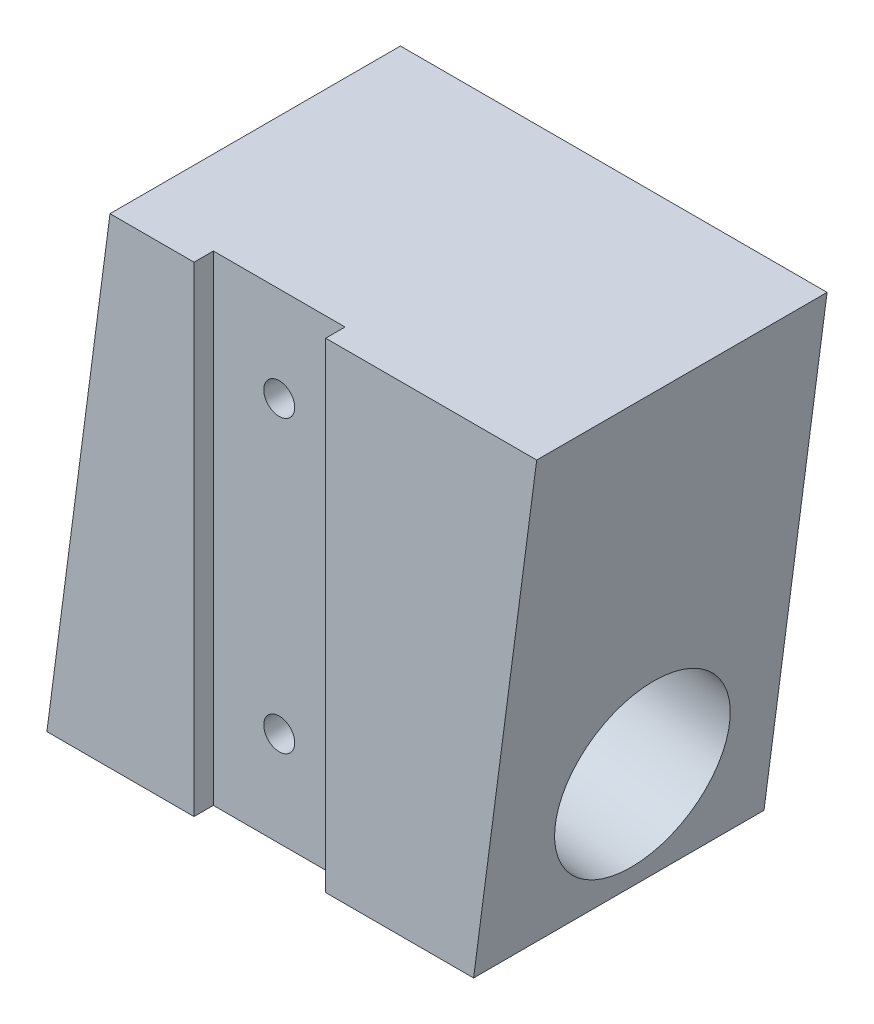
SolidWorks part; units mm, degrees
material "6061 合金"
ref_plane "前视基准面" through (0, 0, 0) normal (0, 0, 1) x (1, 0, 0)
ref_plane "上视基准面" through (0, 0, 0) normal (0, 1, 0) x (1, 0, 0)
ref_plane "右视基准面" through (0, 0, 0) normal (1, 0, 0) x (0, 0, -1)
sketch "草图1" plane through (0, 0, 0) normal (0, 0, 1) x (1, 0, 0)
  line L1 (-19.6362, 9.8181) -> (5.6638, 9.8181)
  line L2 (-19.6362, 9.8181) -> (-19.6362, -14.9819)
  line L3 (-19.6362, -14.9819) -> (5.6638, -14.9819)
  line L4 (5.6638, 9.8181) -> (5.6638, -14.9819)
  dimension "D1" = 24.8
  dimension "D2" = 25.3
extrude "凸台-拉伸1" add sketch "草图1" along normal blind 15
sketch "草图2" plane through (0, 0, 0) normal (0, 0, -1) x (-1, 0, 0)
  line L0 (-5.6638, 9.8181) -> (-2.4038, -14.9819)
  line L1 (19.6362, -14.9819) -> (-5.6638, -14.9819) construction
  line L2 (-2.4038, -14.9819) -> (-5.6638, -14.9819)
  line L3 (-5.6638, -14.9819) -> (-5.6638, 9.8181)
  line L4 (16.3762, 9.8181) -> (19.6362, 9.8181)
  line L5 (-5.6638, 9.8181) -> (19.6362, 9.8181) construction
  line L6 (19.6362, 9.8181) -> (19.6362, -14.9819)
  line L7 (19.6362, -14.9819) -> (16.3762, 9.8181)
  dimension "D1" = 3.26
  dimension "D2" = 3.26
extrude "切除-拉伸1" cut sketch "草图2" against normal up to next
sketch "草图3" plane through (0, -14.9819, 0) normal (0, -1, 0) x (1, 0, 0)
  line L0 (-19.6362, 15) -> (2.4038, 15) construction
  line L1 (-5.2362, 15) -> (-12.0362, 15)
  line L2 (-5.2362, 15) -> (-5.2362, 14)
  line L3 (-5.2362, 14) -> (-12.0362, 14)
  line L4 (-12.0362, 15) -> (-12.0362, 14)
  line L5 (-19.6362, 15) -> (-19.6362, 0) construction
  dimension "D1" = 6.8
  dimension "D2" = 1
  dimension "D3" = 7.6
extrude "切除-拉伸2" cut sketch "草图3" against normal up to next
sketch "草图5" plane through (4.2989, -0.5651, 0) normal (0.9915, -0.1303, 0) x (0, 0, -1)
  line L0 (0, -14.5408) -> (0, 10.4725) construction
  line L1 (-15, -17.4133) -> (0, -17.4133) construction
  circle A0 centre (-7, -9.0133) radius 4.5
  dimension "D1" = 9
  dimension "D2" = 7
  dimension "D3" = 8.4
extrude "切除-拉伸3" cut sketch "草图5" against normal up to next
sketch "草图7" plane through (0, 0, 14) normal (0, 0, 1) x (1, 0, 0)
  line L0 (-5.2362, 9.8181) -> (-5.2362, -14.9819) construction
  line L1 (-5.2362, 9.8181) -> (-12.0362, 9.8181) construction
  circle A0 centre (-8.6362, 4.9181) radius 0.8
  circle A1 centre (-8.6362, -10.0819) radius 0.8
  dimension "D1" = 1.6
  dimension "D2" = 3.4
  dimension "D4" = 4.9
  dimension "D3" = 2
extrude "切除-拉伸4" cut sketch "草图7" against normal blind 6
